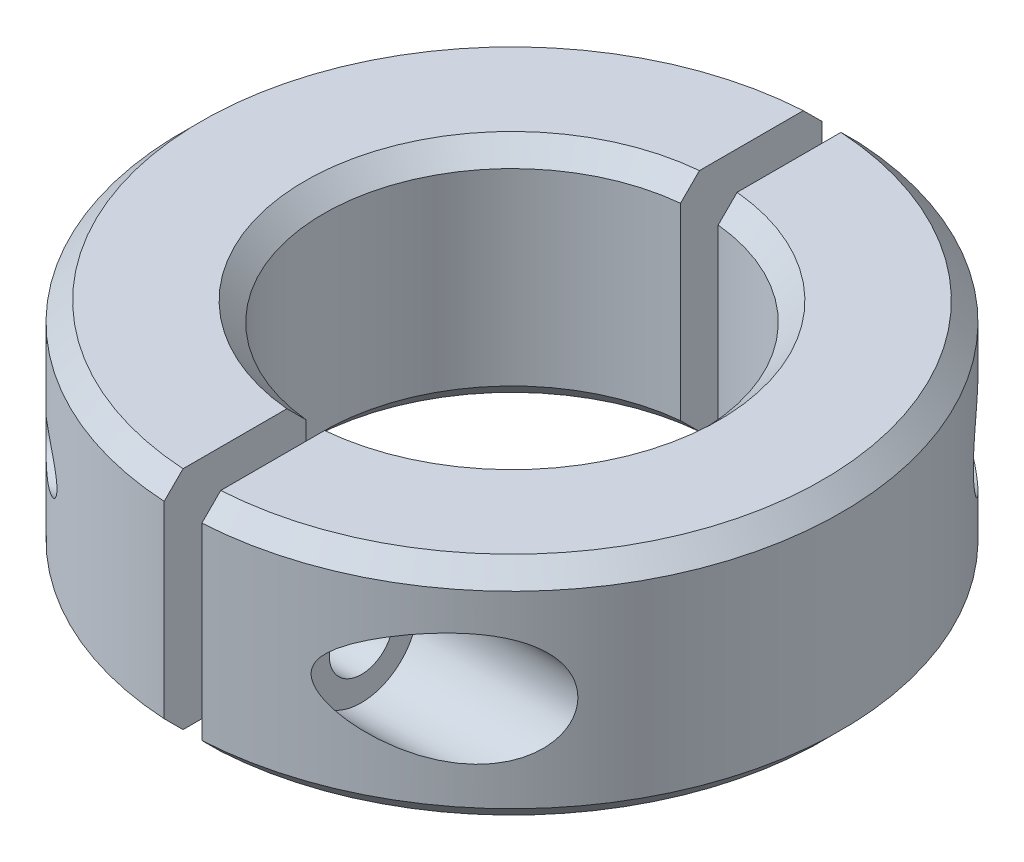
from build123d import *

# Parameters (mm, degrees)
SKETCH_1_R          = 17.5
SKETCH_1_R_2        = 10
EXTRUDE_1_DEPTH     = 6
CHAMFER_1_SIZE      = 1
SKETCH_2_W          = 2
SKETCH_2_H          = 40
CUT_EXTRUDE_1_DEPTH = 28.504545079
SKETCH_11_W         = 1.25
SKETCH_11_H         = 16.5


with BuildPart() as part:
    # 草图1 → 凸台-拉伸1 (new, symmetric)
    with BuildSketch(Plane(origin=(0, 0, 0), x_dir=(1, 0, 0), z_dir=(0, 1, 0))):
        with Locations(Location((0, 0, 0), (0, 0, 270))):
            Circle(SKETCH_1_R)
        with Locations(Location((0, 0, 0), (0, 0, 270))):
            Circle(SKETCH_1_R_2, mode=Mode.SUBTRACT)
    extrude(amount=EXTRUDE_1_DEPTH, both=True)

    # 倒角1
    chamfer_1_edges = [part.edges().sort_by_distance(p)[0] for p in [
        (0, -6, -17.5),
        (0, 6, -17.5),
        (0, -6, -10),
        (0, 6, -10),
    ]]
    chamfer(chamfer_1_edges, length=CHAMFER_1_SIZE)

    # 草图2 → 切除-拉伸1 (cut, through all)
    with BuildSketch(Plane(origin=(0, 6, 0), x_dir=(1, 0, 0), z_dir=(0, 1, 0))):
        Rectangle(SKETCH_2_W, SKETCH_2_H)
    extrude(amount=-CUT_EXTRUDE_1_DEPTH, mode=Mode.SUBTRACT)


with BuildPart() as cut_extrude_1_piece_1:
    # of the separate pieces the step leaves, piece 1, a body of its own (cut_extrude_1_pieces)
    add(part.part.solids().sort_by_distance((-1, -5, -17.47140521))[0])

    # 草图11 → Hole Wizard M3 _1 2 (revolve, cut)
    with BuildSketch(Plane(origin=(-1, 0, -13.5), x_dir=(0, 0, -1), z_dir=(0, 1, 0))):
        with Locations((0.625, 8.25)):
            Rectangle(SKETCH_11_W, SKETCH_11_H)
    hole_wizard_m3_1_2 = revolve(axis=Axis((5.35, 0, -13.5), (-1, 0, 0)), mode=Mode.SUBTRACT)


with BuildPart() as cut_extrude_1_piece_2:
    # of the separate pieces the step leaves, piece 2, a body of its own (cut_extrude_1_pieces)
    add(part.part.solids().sort_by_distance((1, -5, 17.47140521))[0])

    # 草图6 → Hole Wizard M3 _1 (revolve, cut)
    with BuildSketch(Plane(origin=(17.5, 0, -13.5), x_dir=(0, 0, -1), z_dir=(0, 1, 0))):
        Polygon((0, 0), (0, 17.521463052), (1.7, 16.5), (1.7, 12), (3, 12), (3, 0), align=None)
    hole_wizard_m3_1 = revolve(axis=Axis((23.85, 0, -13.5), (-1, 0, 0)), mode=Mode.SUBTRACT)


with BuildPart() as mirror_1_tool:
    # 镜向1: Hole Wizard M3 _1, Hole Wizard M3 _1 2 across plane
    add(hole_wizard_m3_1.mirror(Plane.XY))
    add(hole_wizard_m3_1_2.mirror(Plane.XY))


with BuildPart() as cut_extrude_1_piece_1_1:
    add(cut_extrude_1_piece_1.part)

    # 镜向1: cut by mirror_1_tool
    add(mirror_1_tool.part, mode=Mode.SUBTRACT)


with BuildPart() as cut_extrude_1_piece_2_1:
    add(cut_extrude_1_piece_2.part)

    # 镜向1: cut by mirror_1_tool
    add(mirror_1_tool.part, mode=Mode.SUBTRACT)


solid = Compound([cut_extrude_1_piece_1_1.part, cut_extrude_1_piece_2_1.part])
